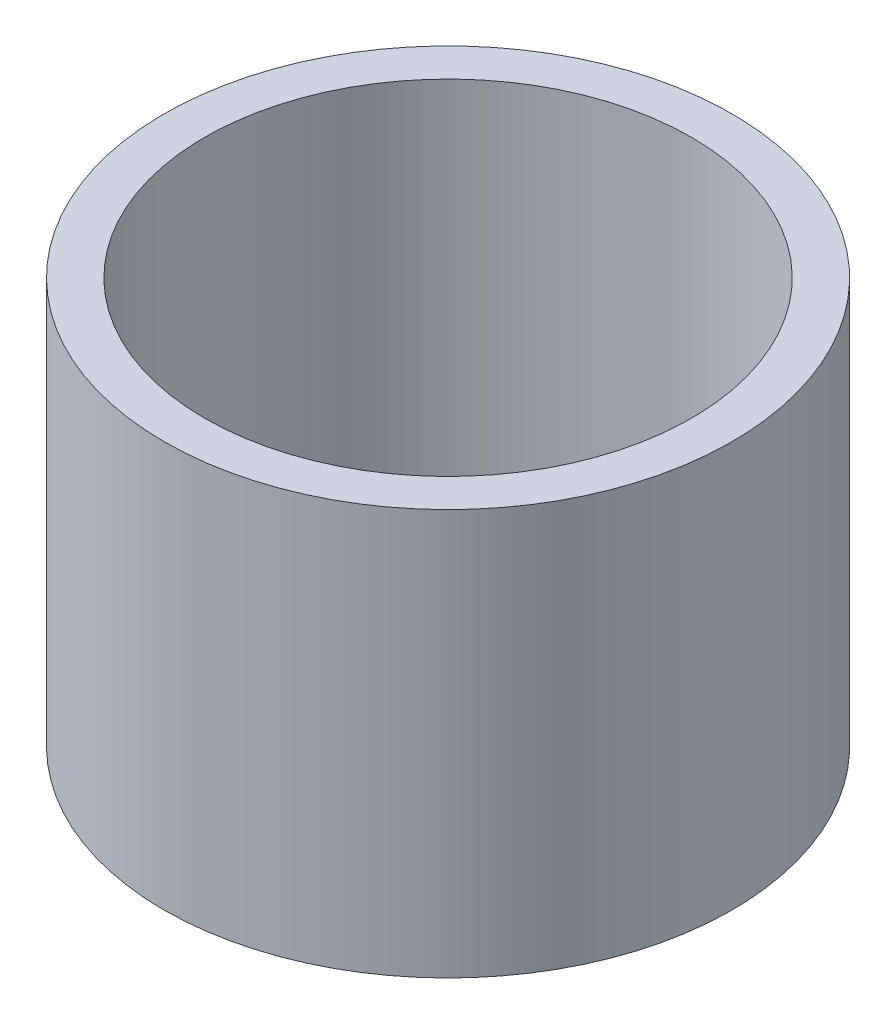
SolidWorks part; units mm, degrees
ref_plane "Front Plane" through (0, 0, 0) normal (0, 0, 1) x (1, 0, 0)
ref_plane "Top Plane" through (0, 0, 0) normal (0, 1, 0) x (1, 0, 0)
ref_plane "Right Plane" through (0, 0, 0) normal (1, 0, 0) x (0, 0, -1)
other "Configuration Table"
sketch "Sketch1" plane through (0, 0, 0) normal (0, 1, 0) x (1, 0, 0)
  circle A0 centre (0, 0) radius 60
  circle A1 centre (0, 0) radius 70
  dimension "D1" = 120
  dimension "D2" = 140
extrude "Boss-Extrude1" add sketch "Sketch1" along normal blind 100
